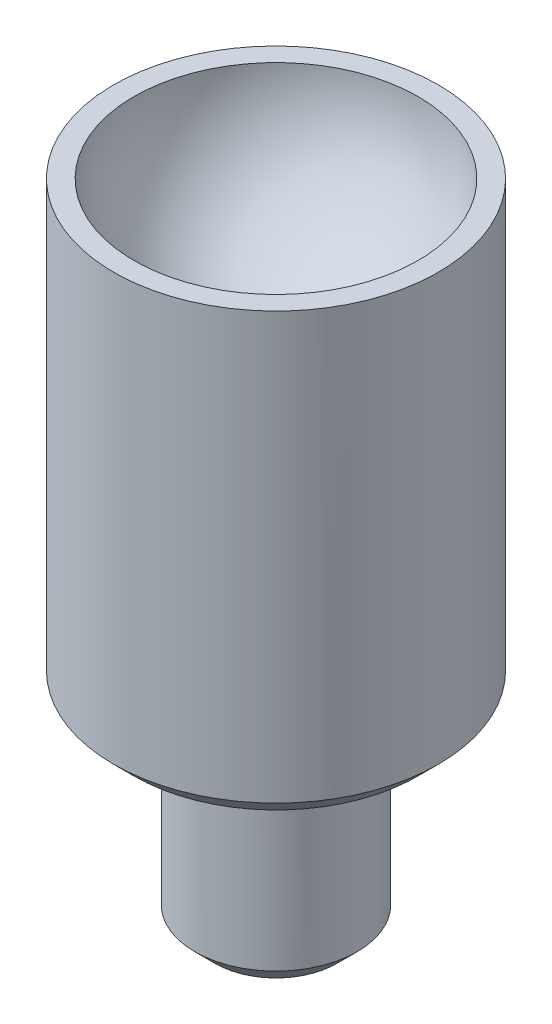
from build123d import *

# Parameters (mm, degrees)
CHAMFER1_SIZE = 1


with BuildPart() as part:
    # Sketch1 → Revolve2 (revolve)
    with BuildSketch(Plane.XY, mode=Mode.PRIVATE) as revolve2_sk:
        with BuildLine():
            Line((-2, 0), (-2, 25.291796068))
            ThreePointArc((-2, 25.291796068), (-5.61248608, 27.816699867), (-7, 32))
            Line((-7, 32), (-8, 32))
            Line((-8, 32), (-8, 10))
            Line((-8, 10), (-4, 10))
            Line((-4, 10), (-4, 0))
            Line((-4, 0), (-2, 0))
        make_face()
    revolve(revolve2_sk.sketch.rotate(Axis((0, 0, 0), (0, 1, 0)), 270), axis=Axis((0, 0, 0), (0, 1, 0)))

    # Chamfer1
    chamfer1_edges = [part.edges().sort_by_distance(p)[0] for p in [
        (0, 10, 8),
        (0, 0, 4),
    ]]
    chamfer(chamfer1_edges, length=CHAMFER1_SIZE)


solid = part.part
